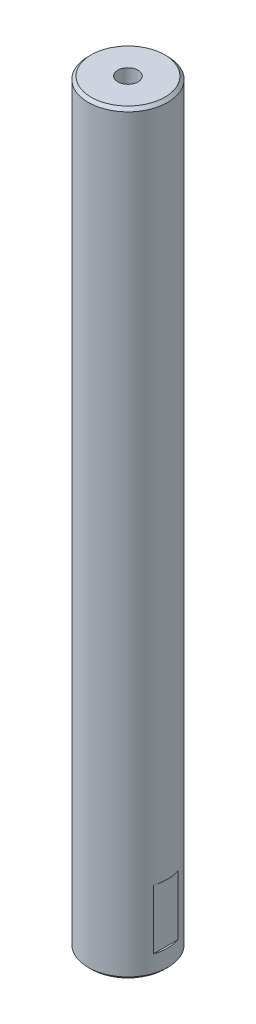
from build123d import *

# Parameters (mm, degrees)
SKETCH1_W               = 20
SKETCH1_H               = 380
CUT_EXTRUDE1_DEPTH      = 344.613267812
CUT_EXTRUDE1_DEPTH_BACK = 344.613267812
SKETCH2_W               = 1
SKETCH2_H               = 30
CHAMFER1_SIZE           = 1.5
M12_TAPPED_HOLE1_D      = 10.2
M12_TAPPED_HOLE1_DEPTH  = 24
M12_TAPPED_HOLE1_TIP    = 3.064389157


with BuildPart() as part:
    # Sketch1 → Revolve1 (revolve)
    with BuildSketch(Plane.XY, mode=Mode.PRIVATE) as revolve1_sk:
        with Locations((-98.74611723, 135.337301587)):
            Rectangle(SKETCH1_W, SKETCH1_H)
    revolve(revolve1_sk.sketch.rotate(Axis((-88.74611723, 325.337301587, 0), (0, -1, 0)), 270), axis=Axis((-88.74611723, 325.337301587, 0), (0, -1, 0)))

    # Sketch2 → Cut-Extrude1 (cut, two sides: drawn at the far end of the back side and taken through both)
    with BuildSketch(Plane.XY.offset(-CUT_EXTRUDE1_DEPTH_BACK)):
        with Locations((-108.24611723, -29.662698413)):
            Rectangle(SKETCH2_W, SKETCH2_H)
        with Locations((-69.24611723, -29.662698413)):
            Rectangle(SKETCH2_W, SKETCH2_H)
    extrude(amount=CUT_EXTRUDE1_DEPTH + CUT_EXTRUDE1_DEPTH_BACK, mode=Mode.SUBTRACT)

    # Chamfer1
    chamfer1_edges = [part.edges().sort_by_distance(p)[0] for p in [
        (-88.74611723, -54.662698413, -20),
        (-88.74611723, 325.337301587, -20),
    ]]
    chamfer(chamfer1_edges, length=CHAMFER1_SIZE)

    # M12 Tapped Hole1
    with Locations(Plane(origin=(0, 325.337301587, 0), x_dir=(1, 0, 0), z_dir=(0, 1, 0))):
        with Locations((-88.74611723, 0)):
            Hole(M12_TAPPED_HOLE1_D / 2, depth=M12_TAPPED_HOLE1_DEPTH)
            with Locations((0, 0, -(M12_TAPPED_HOLE1_DEPTH + M12_TAPPED_HOLE1_TIP / 2))):  # 118° drill point
                Cone(0, M12_TAPPED_HOLE1_D / 2, M12_TAPPED_HOLE1_TIP, mode=Mode.SUBTRACT)


solid = part.part
